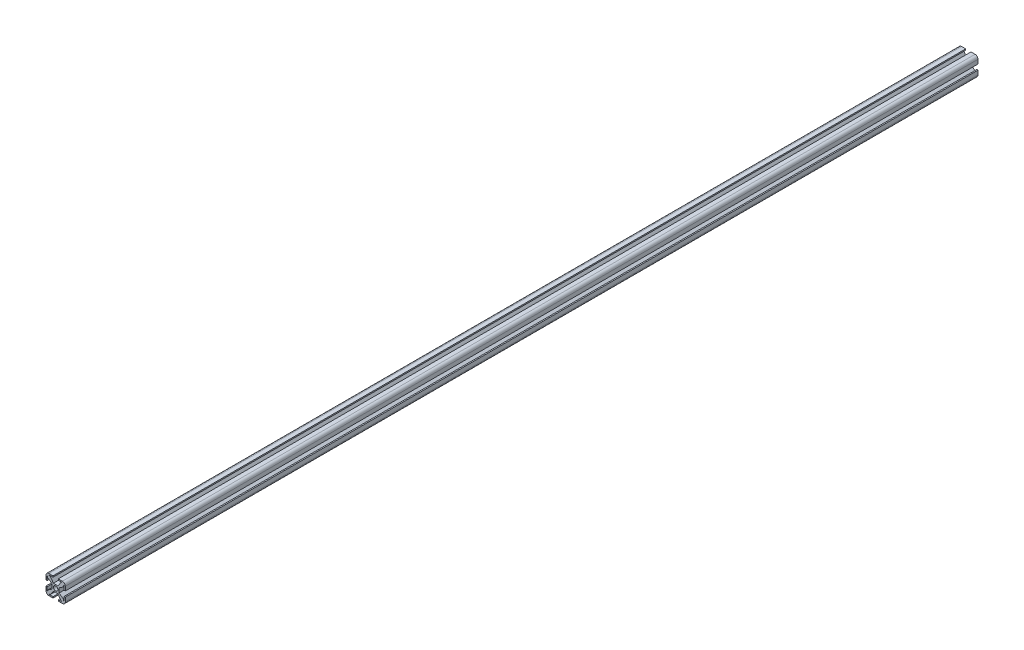
from build123d import *

# Parameters (mm, degrees)
SKETCH_1_W               = 30
SKETCH_1_H               = 30
EXTRUDE_1_DEPTH          = 710
FILLET_1_R               = 4.5
SKETCH_2_W               = 8.2
SKETCH_2_H               = 0.3
SKETCH_2_H_2             = 1.9
SKETCH_2_R               = 3.4
CUT_EXTRUDE_1_DEPTH      = 1421.158441865
PATTERN_CIRCULAR_1_COUNT = 4


with BuildPart() as part:
    # 草图1 → 凸台-拉伸1 (new, symmetric)
    with BuildSketch(Plane.XY):
        Rectangle(SKETCH_1_W, SKETCH_1_H)
    extrude(amount=EXTRUDE_1_DEPTH, both=True)

    # 圆角1
    fillet_1_edges = [part.edges().sort_by_distance(p)[0] for p in [
        (-15, 15, 0),
        (15, 15, 0),
        (15, -15, 0),
        (-15, -15, 0),
    ]]
    fillet(fillet_1_edges, radius=FILLET_1_R)

    # 草图2 → 切除-拉伸1 (cut, through all)
    with BuildSketch(Plane.XY.offset(710)):
        with Locations((0, 12.95)):
            Rectangle(SKETCH_2_W, SKETCH_2_H)
        with Locations((0, 14.05)):
            Rectangle(SKETCH_2_W, SKETCH_2_H_2)
        Polygon((10.25, 13.1), (4.1, 13.1), (4.1, 12.8), (-4.1, 12.8), (-4.1, 13.1), (-10.25, 13.1), (-10.25, 12.5), (-8.429704265, 12.5), (8.429704265, 12.5), (10.25, 12.5), align=None)
        Polygon((3.479704265, 5.3), (8.429704265, 12.5), (-8.429704265, 12.5), (-3.479704265, 5.3), align=None)
        Circle(SKETCH_2_R)
    cut_extrude_1 = extrude(amount=-CUT_EXTRUDE_1_DEPTH, mode=Mode.SUBTRACT)

    # 阵列(圆周)1: 切除-拉伸1 ×4 about axis
    pattern_circular_1_axis = Axis((0, 0, 0), (0, 0, 1))
    for i in range(1, PATTERN_CIRCULAR_1_COUNT):
        add(cut_extrude_1.rotate(pattern_circular_1_axis, i * 360 / PATTERN_CIRCULAR_1_COUNT), mode=Mode.SUBTRACT)


solid = part.part
